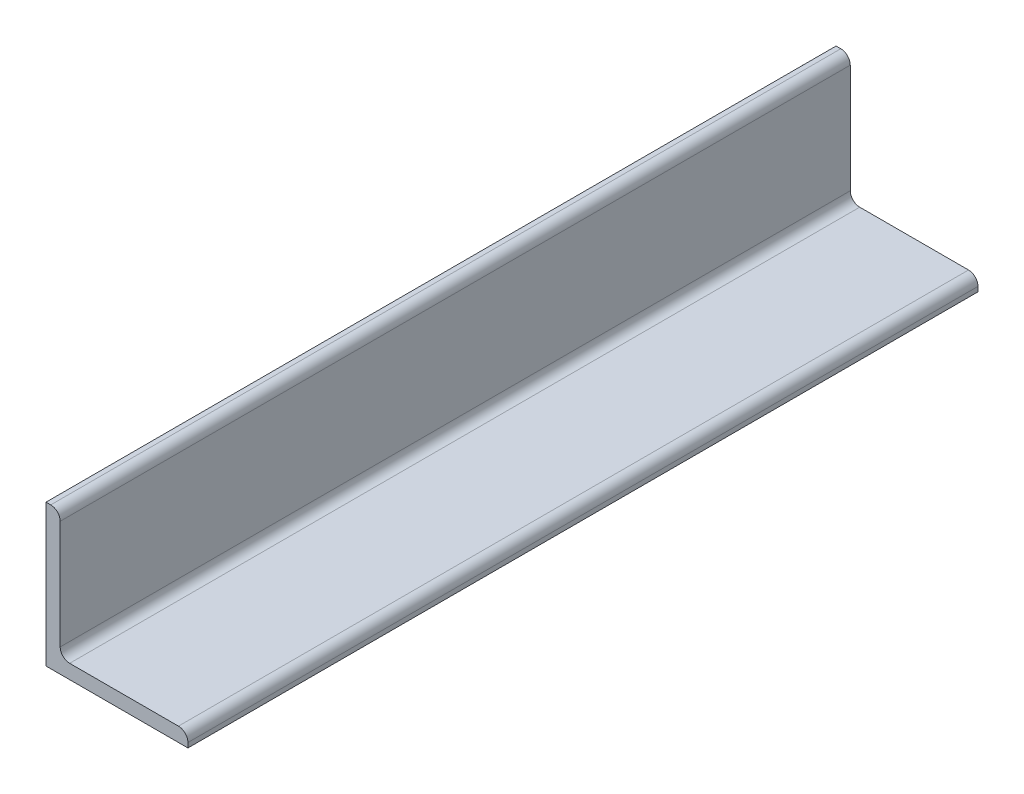
from build123d import *

# Parameters (mm, degrees)
BOSS_EXTRUDE1_DEPTH = 167


with BuildPart() as part:
    # Sketch1 → Boss-Extrude1 (new body)
    with BuildSketch(Plane.XY):
        with BuildLine():
            Line((0, 0), (30, 0))
            Line((30, 0), (30, 1))
            ThreePointArc((30, 1), (29.414213562, 2.414213562), (28, 3))
            Line((28, 3), (5, 3))
            ThreePointArc((5, 3), (3.585786438, 3.585786438), (3, 5))
            Line((3, 5), (3, 28))
            ThreePointArc((3, 28), (2.414213562, 29.414213562), (1, 30))
            Line((1, 30), (0, 30))
            Line((0, 30), (0, 0))
        make_face()
    extrude(amount=BOSS_EXTRUDE1_DEPTH)


solid = part.part
